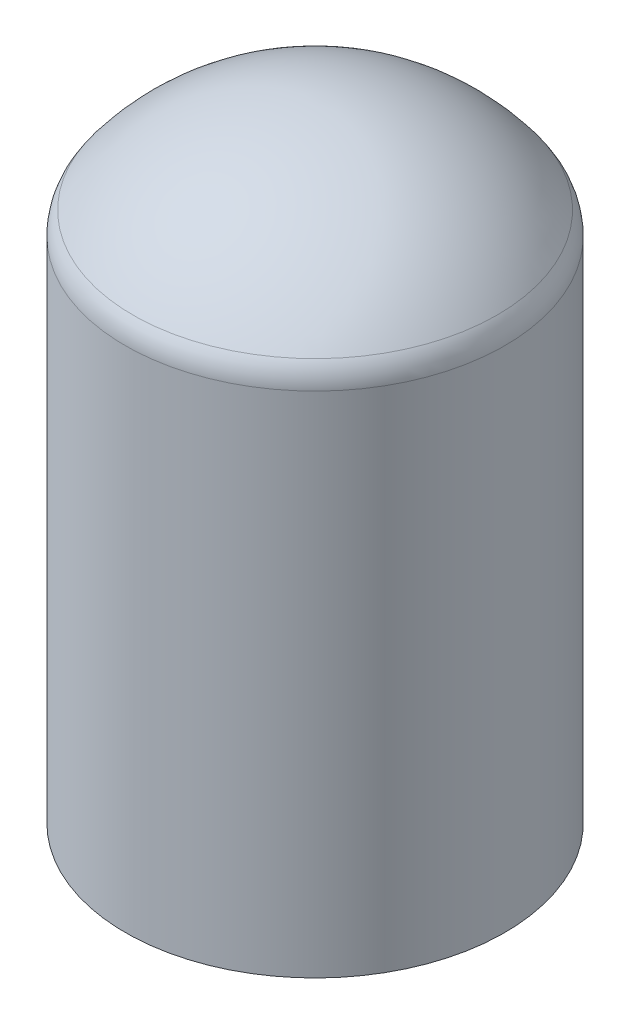
from build123d import *

# Parameters (mm, degrees)
FILLET1_R = 50
SHELL1_T  = -70


with BuildPart() as part:
    # Sketch1 → Revolve1 (revolve)
    with BuildSketch(Plane.XY, mode=Mode.PRIVATE) as revolve1_sk:
        with BuildLine():
            Line((0, 0), (0, 700))
            Line((0, 700), (0, 820))
            ThreePointArc((0, 820), (141.863716546, 784.338203685), (250, 685.831239518))
            Line((250, 685.831239518), (250, 0))
            Line((250, 0), (0, 0))
        make_face()
    revolve(revolve1_sk.sketch.rotate(Axis((0, 0, 0), (0, 1, 0)), 90), axis=Axis((0, 0, 0), (0, 1, 0)))

    # Fillet1
    fillet1_edges = [part.edges().sort_by_distance(p)[0] for p in [
        (0, 685.831239518, 250),
    ]]
    fillet(fillet1_edges, radius=FILLET1_R)

    # Shell1
    shell1_openings = [part.faces().sort_by_distance(p)[0] for p in [
        (0, 0, 0),
    ]]
    offset(amount=SHELL1_T, openings=shell1_openings, kind=Kind.INTERSECTION)


solid = part.part
